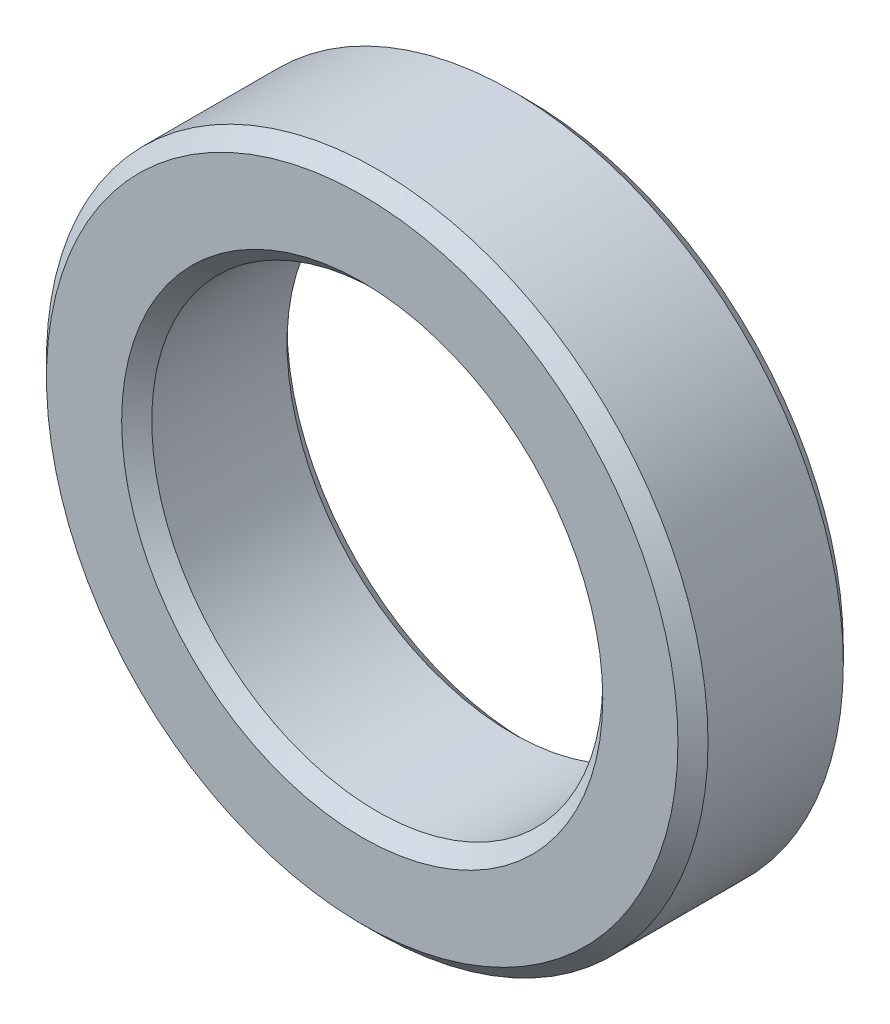
SolidWorks part; units mm, degrees
material "Plain carbon steel"
ref_plane "Front Plane" through (0, 0, 0) normal (0, 0, 1) x (1, 0, 0)
ref_plane "Top Plane" through (0, 0, 0) normal (0, 1, 0) x (1, 0, 0)
ref_plane "Right Plane" through (0, 0, 0) normal (1, 0, 0) x (0, 0, -1)
sketch "Sketch1" plane through (0, 0, 0) normal (0, 0, 1) x (1, 0, 0)
  circle A0 centre (0, 0) radius 7.5
  circle A1 centre (0, 0) radius 11
  dimension "D1" = 15
  dimension "D2" = 22
extrude "Boss-Extrude1" add sketch "Sketch1" along normal blind 5.5
chamfer "Chamfer1" distance 0.5 angle 45 4 edges at (11, 0, 0) (11, 0, 5.5) (7.5, 0, 0) (7.5, 0, 5.5)
